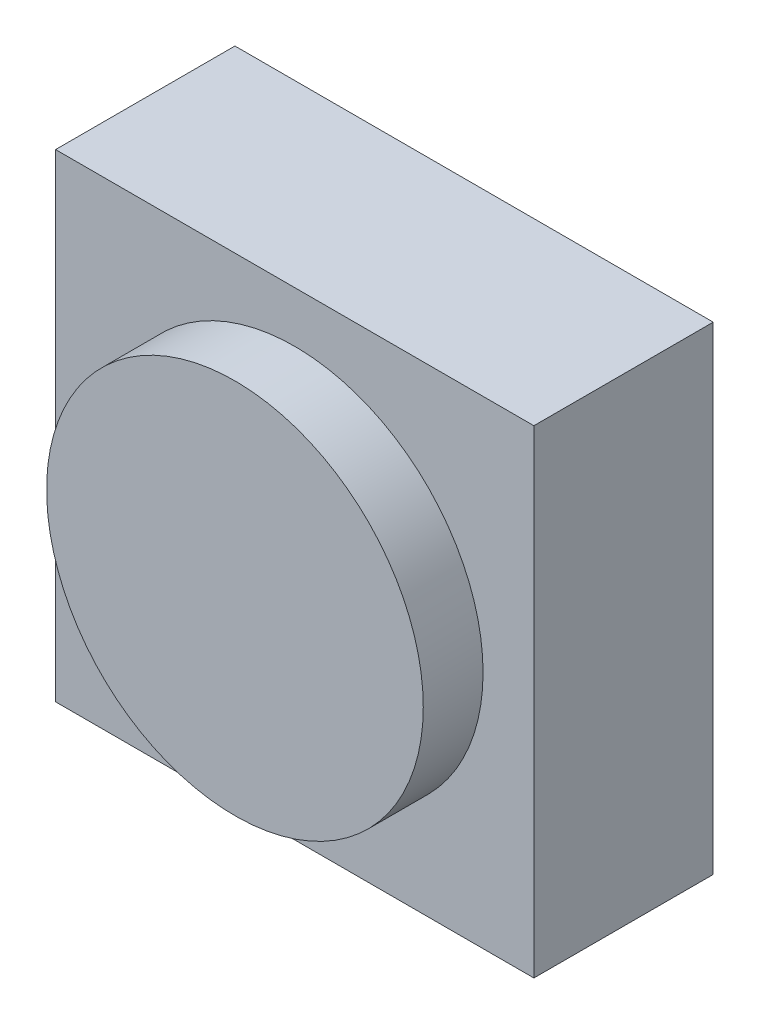
SolidWorks part; units mm, degrees
ref_plane "前视基准面" through (0, 0, 0) normal (0, 0, 1) x (1, 0, 0)
ref_plane "上视基准面" through (0, 0, 0) normal (0, 1, 0) x (1, 0, 0)
ref_plane "右视基准面" through (0, 0, 0) normal (1, 0, 0) x (0, 0, -1)
other "Configuration Table"
sketch "草图1" plane through (0, 0, 0) normal (0, 0, 1) x (1, 0, 0)
  line L1 (-40, -40) -> (40, -40)
  line L2 (-40, -40) -> (-40, 40)
  line L3 (-40, 40) -> (40, 40)
  line L4 (40, -40) -> (40, 40)
  line L5 (0, 40) -> (0, -40) construction
  line L6 (-40, 0) -> (40, 0) construction
  point P0 (0, 0)
  dimension "D1" = 80
  dimension "D2" = 80
extrude "凸台-拉伸1" add sketch "草图1" along normal blind 30
sketch "草图2" plane through (0, 0, 30) normal (0, 0, 1) x (1, 0, 0)
  circle A0 centre (0, 0) radius 31.5
  dimension "D1" = 63
extrude "凸台-拉伸2" add sketch "草图2" along normal blind 10
